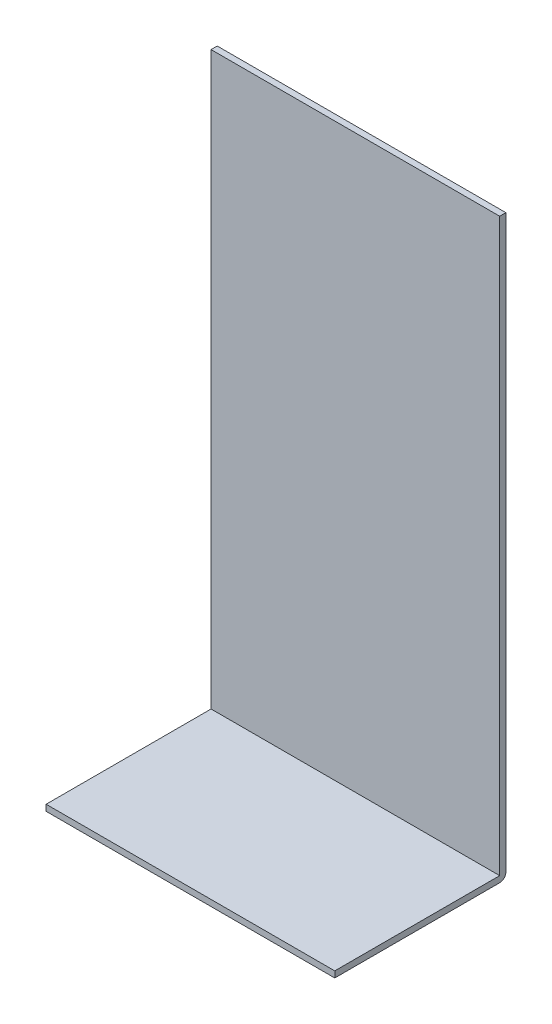
SolidWorks part; units mm, degrees
ref_plane "前视基准面" through (0, 0, 0) normal (0, 0, 1) x (1, 0, 0)
ref_plane "上视基准面" through (0, 0, 0) normal (0, 1, 0) x (1, 0, 0)
ref_plane "右视基准面" through (0, 0, 0) normal (1, 0, 0) x (0, 0, -1)
sketch "草图1" plane through (0, 0, 0) normal (0, 0, 1) x (1, 0, 0)
  line L0 (0, 0) -> (140, 0)
  line L1 (140, 0) -> (140, -280)
  line L2 (140, -280) -> (0, -280)
  line L3 (0, -280) -> (0, 0)
extrude "凸台-拉伸1" add sketch "草图1" along normal blind 3
sketch "草图2" plane through (0, 0, 3) normal (0, 0, 1) x (1, 0, 0)
  line L0 (140, -280) -> (140, -277)
  line L1 (140, -280) -> (140, 0) construction
  line L2 (140, -277) -> (0, -277)
  line L3 (0, 0) -> (0, -280) construction
  line L4 (0, -277) -> (0, -280)
  line L5 (0, -280) -> (140, -280)
extrude "凸台-拉伸2" add sketch "草图2" along normal blind 80
fillet "圆角1" radius 3 1 edges at (70, -280, 0)
